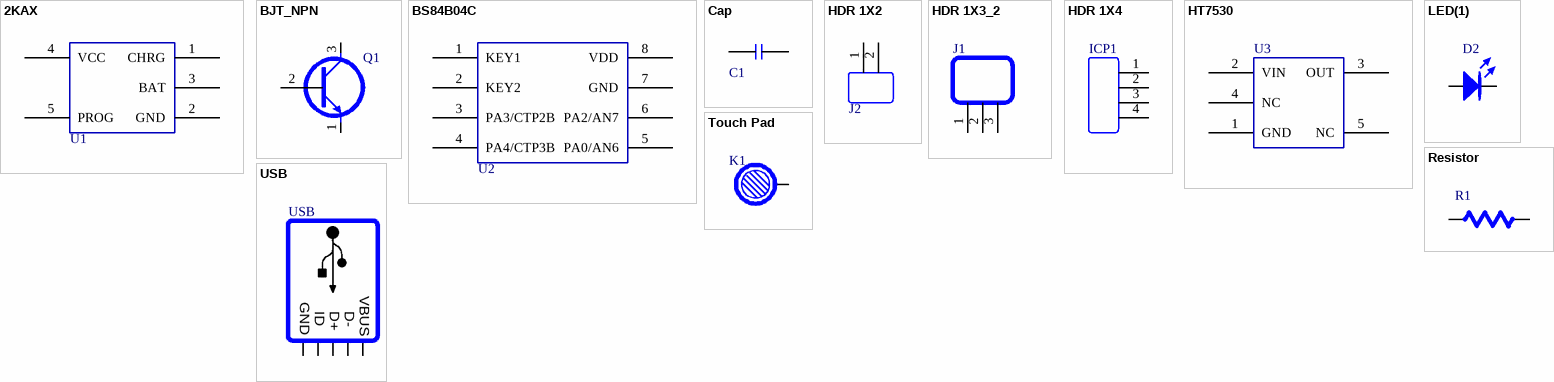
[diagram p0: symbols 2KAX to USB]
# Altium schematic symbol library MISC64789-3.SchLib: 12 symbols
Pins are listed as number, name and electrical type; pins without a type are passive.


## 2KAX
designator U1
footprint SOT23 PIN-5
pins: 1 CHRG, 2 GND, 3 BAT, 4 VCC, 5 PROG

## BJT_NPN
designator Q1
NPN Bipolar Transistor
footprint SOT23_BJT_NPN
pins: 1 E, 2 B, 3 C

## BS84B04C
designator U2
footprint SOP8 (SOP8,Pitch=1.27mm,LxWxH=5.15x6.2x1.5.)
pins: 1 KEY1, 2 KEY2, 3 PA3/CTP2B, 4 PA4/CTP3B, 5 PA0/AN6, 6 PA2/AN7, 7 GND, 8 VDD

## Cap
designator C1
footprint C 0603 (SMD 06003 2.5x1 mm)
footprint C 1206 (SMD 1206 5x1.5 mm)
footprint C 0402 (C 0402, L=1.9(mm),W=0.5,space=0.635.)
pins: 1, 2

## HDR 1X2
designator J2
footprint HDR 1X2 Pitch 2.5mm (Header; 2 Position; Pitch 2.5mm)
pins: 1, 2

## HDR 1X3_2
designator J1
footprint HDR1X3 (Connector; Header; 3 Position)
footprint 焊盤
pins: 1, 2, 3

## HDR 1X4
designator ICP1
footprint HDR 1x4(2.54)
pins: 1, 2, 3, 4

## HT7530
designator U3
footprint SOT23 PIN-5
footprint SOT23 PIN-5
pins: 1 GND, 2 VIN, 3 OUT, 4 NC, 5 NC

## LED(1)
designator D2
Typical INFRARED GaAs LED
footprint LED-0 (LED; 2 Leads)
simulation model LED0 (Diode)
footprint LED3M
footprint LED_0603
pins: 1 A, 2 K

## Resistor
designator R1
Resisitor
footprint R 0603 (SMD 0603 2.5x1 mm)
pins: 1, 2

## Touch Pad
designator K1
footprint KEY
pins: 1

## USB
designator USB
Mini/Micro
footprint USB_MINI
footprint MicroUSB
footprint Micro USB_02
pins: 1 VDD, 2 D-, 3 D+, 4 GND (power), 5 GND (power)